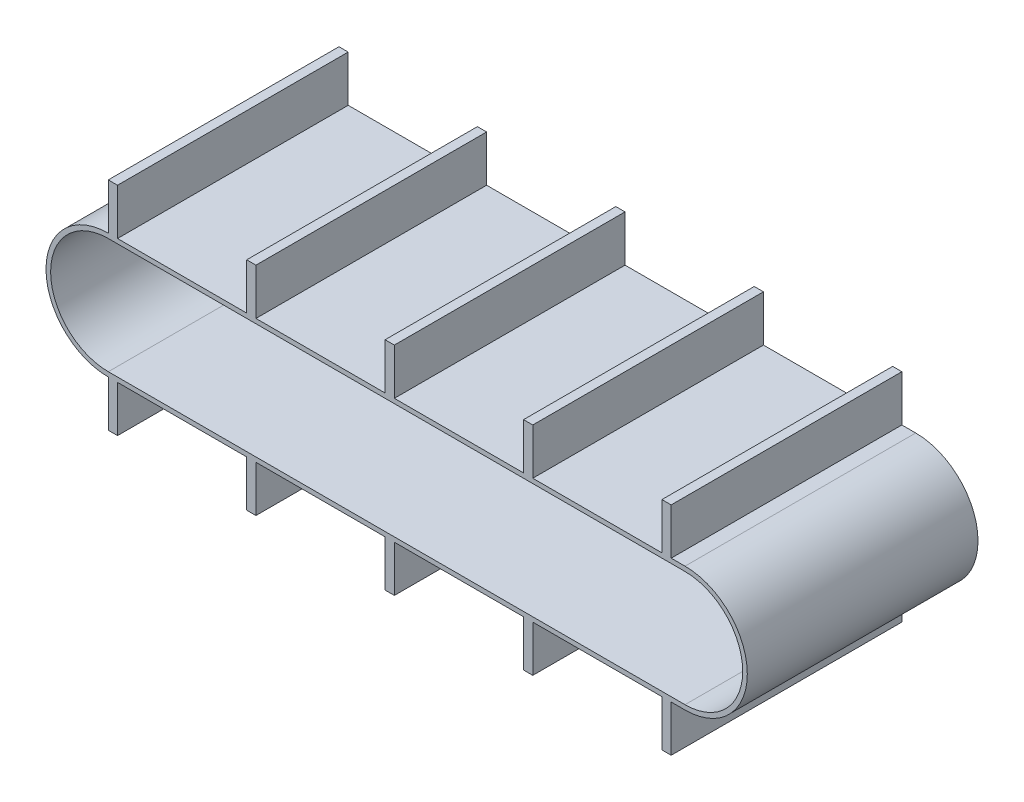
SolidWorks part; units mm, degrees
ref_plane "前视基准面" through (0, 0, 0) normal (0, 0, 1) x (1, 0, 0)
ref_plane "上视基准面" through (0, 0, 0) normal (0, 1, 0) x (1, 0, 0)
ref_plane "右视基准面" through (0, 0, 0) normal (1, 0, 0) x (0, 0, -1)
sketch "草图1" plane through (0, 0, 0) normal (0, 0, 1) x (1, 0, 0)
  line L0 (0, 0) -> (250, 0) construction
  line L1 (0, 25) -> (250, 25)
  line L2 (0, -25) -> (250, -25)
  line L3 (0, 27) -> (250, 27)
  line L4 (0, -27) -> (250, -27)
  arc A0 (0, 25) -> (0, -25) centre (0, 0) ccw
  arc A1 (250, -25) -> (250, 25) centre (250, 0) ccw
  arc A2 (250, -27) -> (250, 27) centre (250, 0) ccw
  arc A3 (0, 27) -> (0, -27) centre (0, 0) ccw
  point P3 (125, 0)
  dimension "D2" = 25
  dimension "D1" = 250
  dimension "D3" = 2
extrude "凸台-拉伸1" add sketch "草图1" along normal blind 100
sketch "草图2" plane through (0, 0, 100) normal (0, 0, 1) x (1, 0, 0)
  line L1 (0, 27) -> (4, 27)
  line L2 (0, 27) -> (0, 47)
  line L3 (0, 47) -> (4, 47)
  line L4 (4, 27) -> (4, 47)
  dimension "D1" = 4
  dimension "D2" = 20
extrude "凸台-拉伸2" add sketch "草图2" against normal up to surface (100 mm away) up to face at (125, 0, 0)
pattern_linear "阵列(线性)1" count 5 spacing 60 along (1, 0, 0) of "凸台-拉伸2"
sketch "草图3" plane through (0, 0, 100) normal (0, 0, 1) x (1, 0, 0)
  line L1 (0, -27) -> (4, -27)
  line L2 (0, -27) -> (0, -47)
  line L3 (0, -47) -> (4, -47)
  line L4 (4, -27) -> (4, -47)
  dimension "D1" = 20
  dimension "D2" = 4
extrude "凸台-拉伸3" add sketch "草图3" against normal up to surface (100 mm away) up to face at (127.8261, 31, 0)
pattern_linear "阵列(线性)2" count 5 spacing 60 along (1, 0, 0) of "凸台-拉伸3"
